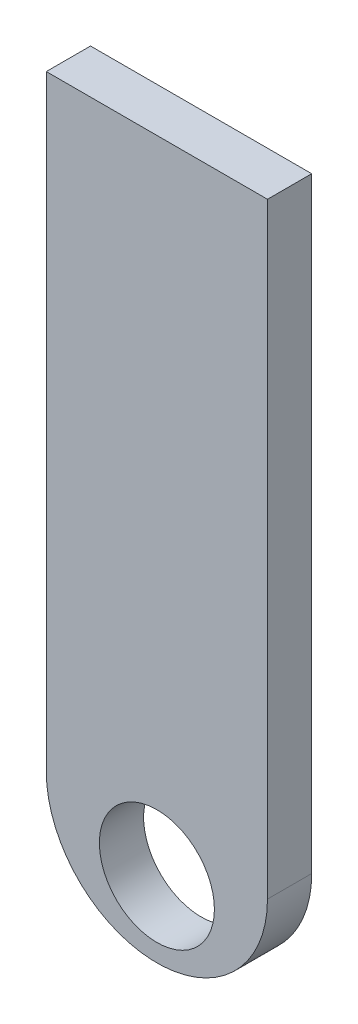
from build123d import *

# Parameters (mm, degrees)
BOSS_EXTRUDE1_DEPTH = 10
SKETCH2_R           = 13
CUT_EXTRUDE1_DEPTH  = 140.620915339


with BuildPart() as part:
    # Sketch1 → Boss-Extrude1 (new body)
    with BuildSketch(Plane.XY):
        with BuildLine():
            Line((-25, 0), (-25, 137))
            Line((-25, 137), (25, 137))
            Line((25, 137), (25, 0))
            ThreePointArc((25, 0), (0, -25), (-25, 0))
        make_face()
    extrude(amount=BOSS_EXTRUDE1_DEPTH)

    # Sketch2 → Cut-Extrude1 (cut, through all)
    with BuildSketch(Plane.XY.offset(10)):
        with Locations((0, -8)):
            Circle(SKETCH2_R)
    extrude(amount=-CUT_EXTRUDE1_DEPTH, mode=Mode.SUBTRACT)


solid = part.part
